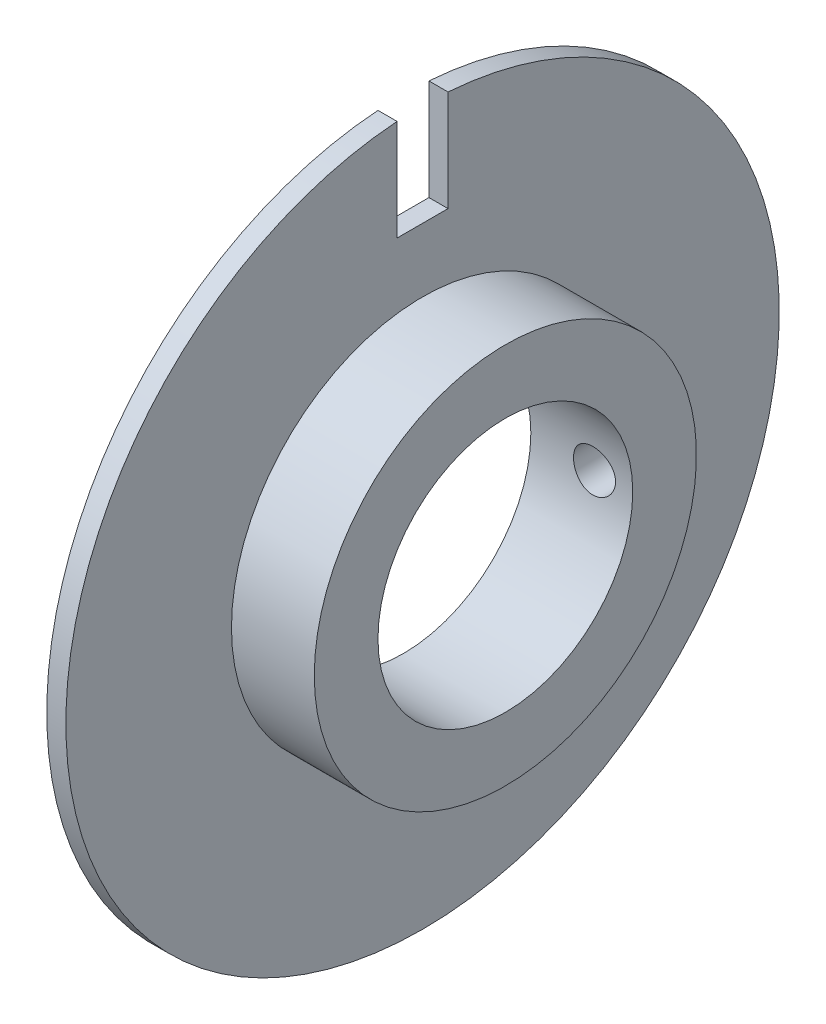
from build123d import *

# Parameters (mm, degrees)
CUT_EXTRUDE1_REACH     = 42.398
SKETCH2_W              = 4
SKETCH2_H              = 9.816803941
M4_TAPPED_HOLE1_REACH  = 53.556
M4_TAPPED_HOLE1_BORE_R = 1.65


with BuildPart() as part:
    # Sketch1 → Revolve1 (revolve)
    with BuildSketch(Plane.XY, mode=Mode.PRIVATE) as revolve1_sk:
        Polygon((0, 10), (8, 10), (8, 15), (1.5, 15), (1.5, 28), (0, 28), align=None)
    revolve(revolve1_sk.sketch.rotate(Axis((0, 0, 0), (1, 0, 0)), 90), axis=Axis((0, 0, 0), (1, 0, 0)))

    # Sketch2 → Cut-Extrude1 (cut, up to next)
    with BuildSketch(Plane.ZY, mode=Mode.PRIVATE) as cut_extrude1_sk1:
        with Locations((0, 24.908401971)):
            Rectangle(SKETCH2_W, SKETCH2_H)
    cut_extrude1_tool1 = extrude(cut_extrude1_sk1.sketch, amount=-CUT_EXTRUDE1_REACH, mode=Mode.PRIVATE) & part.part
    add(cut_extrude1_tool1.solids().sort_by_distance((0, 24.908402, 0))[0], mode=Mode.SUBTRACT)

    # M4 Tapped Hole1 bore (on position points) → M4 Tapped Hole1 (cut, up to next)
    with BuildSketch(Plane(origin=(5, 0, -15), x_dir=(0, -1, 0), z_dir=(0, 0, -1)), mode=Mode.PRIVATE) as m4_tapped_hole1_sk1:
        Circle(M4_TAPPED_HOLE1_BORE_R)
    m4_tapped_hole1_tool1 = extrude(m4_tapped_hole1_sk1.sketch, amount=-M4_TAPPED_HOLE1_REACH, mode=Mode.PRIVATE) & part.part
    add(m4_tapped_hole1_tool1.solids().sort_by_distance((5, 0, -15))[0], mode=Mode.SUBTRACT)


solid = part.part
